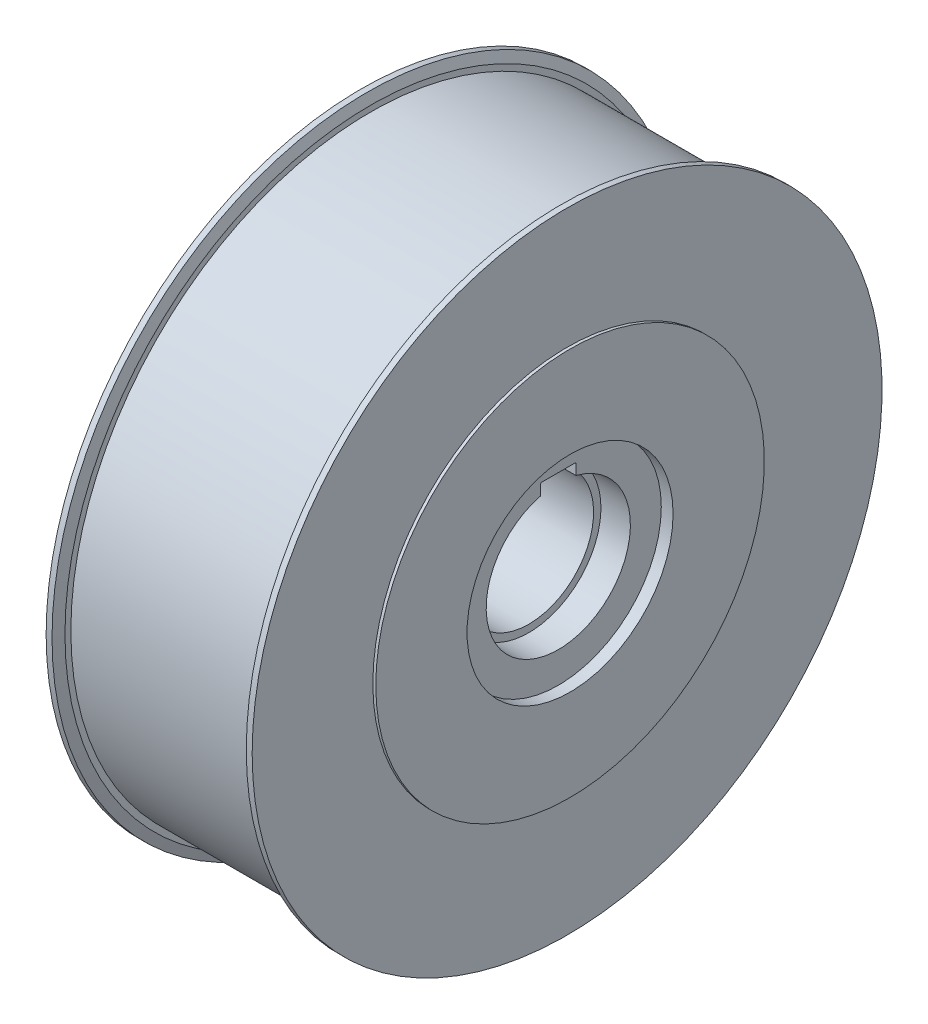
from build123d import *

# Parameters (mm, degrees)
SKETCH2_R          = 17.5
CUT_EXTRUDE1_DEPTH = 2
CUT_EXTRUDE2_DEPTH = 83.948779376
SKETCH4_R          = 12.25
CUT_EXTRUDE3_DEPTH = 5
FILLET1_R          = 0.2


with BuildPart() as part:
    # Sketch1 → Revolve1 (revolve)
    with BuildSketch(Plane.XY, mode=Mode.PRIVATE) as revolve1_sk:
        Polygon((-18, 0), (-18, 33), (-17.5, 33), (-17.5, 53.5), (-16.5, 53.5), (-15.9, 51.9), (-15.9, 50.9), (15.9, 50.9), (15.9, 51.9), (16.5, 53.5), (17.5, 53.5), (17.5, 33), (18, 33), (18, 0), align=None)
    revolve(revolve1_sk.sketch.rotate(Axis((-18, 0, 0), (1, 0, 0)), 90), axis=Axis((-18, 0, 0), (1, 0, 0)))

    # Sketch2 → Cut-Extrude1 (cut)
    with BuildSketch(Plane(origin=(18, 0, 0), x_dir=(0, 0, -1), z_dir=(1, 0, 0))):
        Circle(SKETCH2_R)
    extrude(amount=-CUT_EXTRUDE1_DEPTH, mode=Mode.SUBTRACT)

    # Sketch3 → Cut-Extrude2 (cut, through all)
    with BuildSketch(Plane(origin=(16, 0, 0), x_dir=(0, 0, -1), z_dir=(1, 0, 0))):
        with BuildLine():
            Line((3, 10.583005244), (3, 13.8))
            Line((3, 13.8), (-3, 13.8))
            Line((-3, 13.8), (-3, 10.583005244))
            ThreePointArc((-3, 10.583005244), (0, -11), (3, 10.583005244))
        make_face()
    extrude(amount=-CUT_EXTRUDE2_DEPTH, mode=Mode.SUBTRACT)

    # Sketch4 → Cut-Extrude3 (cut)
    with BuildSketch(Plane(origin=(16, 0, 0), x_dir=(0, 0, -1), z_dir=(1, 0, 0))):
        Circle(SKETCH4_R)
    extrude(amount=-CUT_EXTRUDE3_DEPTH, mode=Mode.SUBTRACT)

    # Fillet1
    fillet1_edges = [part.edges().sort_by_distance(p)[0] for p in [
        (-1, 13.8, 3),
        (-1, 13.8, -3),
    ]]
    fillet(fillet1_edges, radius=FILLET1_R)


solid = part.part
